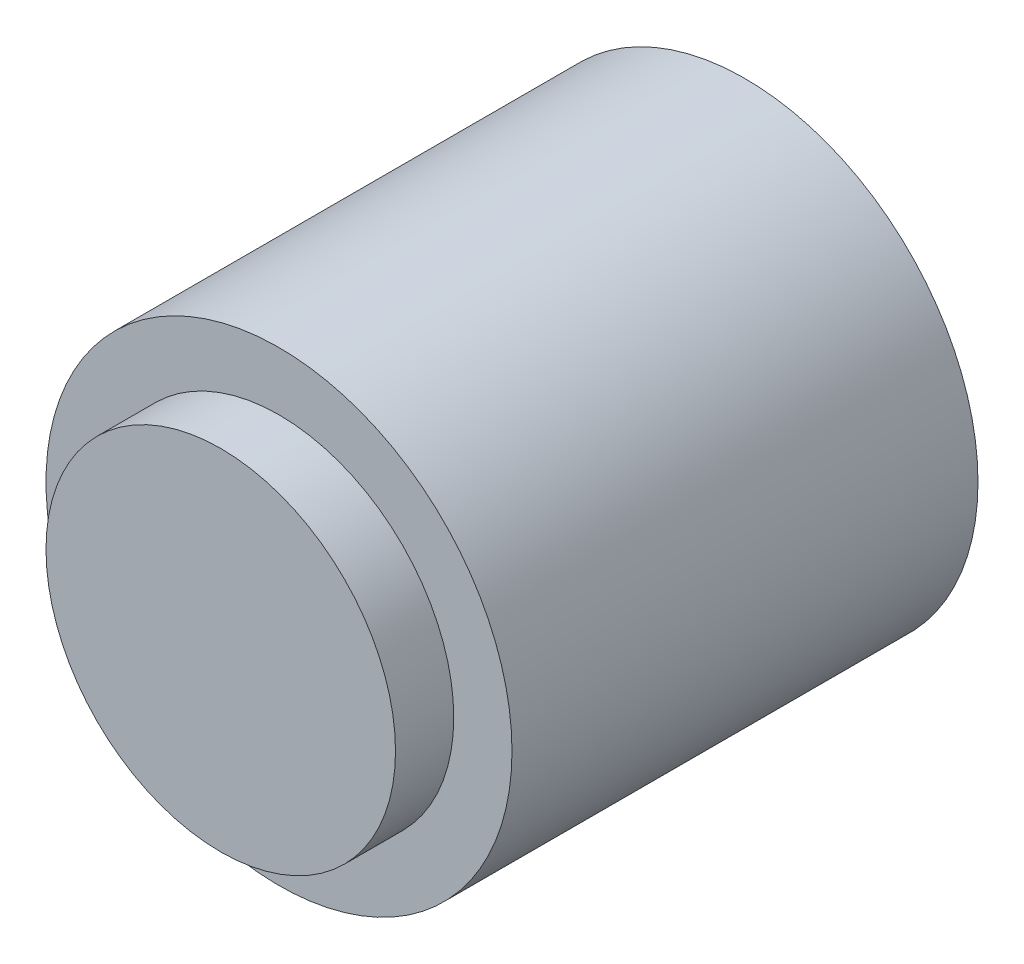
SolidWorks part; units mm, degrees
ref_plane "Front Plane" through (0, 0, 0) normal (0, 0, 1) x (1, 0, 0)
ref_plane "Top Plane" through (0, 0, 0) normal (0, 1, 0) x (1, 0, 0)
ref_plane "Right Plane" through (0, 0, 0) normal (1, 0, 0) x (0, 0, -1)
sketch "Sketch1" plane through (0, 0, 0) normal (0, 0, 1) x (1, 0, 0)
  circle A0 centre (0, 0) radius 20
  dimension "D1" = 40
extrude "Boss-Extrude1" add sketch "Sketch1" along normal blind 40
sketch "Sketch2" plane through (0, 0, 40) normal (0, 0, 1) x (1, 0, 0)
  circle A0 centre (0, 0) radius 15
  dimension "D1" = 30
extrude "Boss-Extrude2" add sketch "Sketch2" along normal blind 5
